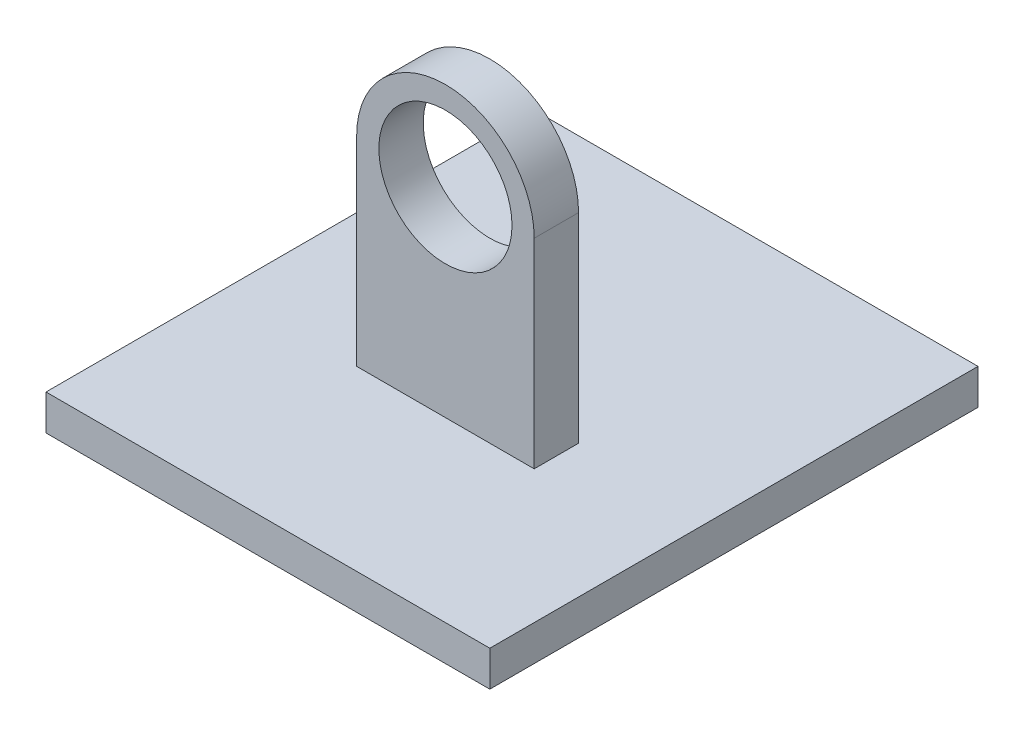
SolidWorks part; units mm, degrees
ref_plane "Front Plane" through (0, 0, 0) normal (0, 0, 1) x (1, 0, 0)
ref_plane "Top Plane" through (0, 0, 0) normal (0, 1, 0) x (1, 0, 0)
ref_plane "Right Plane" through (0, 0, 0) normal (1, 0, 0) x (0, 0, -1)
sketch "Sketch1" plane through (0, 0, 0) normal (0, 0, 1) x (1, 0, 0)
  line L0 (119, -40) -> (119, -108.669) construction
  line L1 (134, -40) -> (134, -80) construction
  line L2 (104, -40) -> (104, -80) construction
  line L3 (134, -80) -> (104, -80) construction
  line L4 (164, -80) -> (74, -80) construction
  line L5 (139, -40) -> (139, -85)
  line L6 (139, -85) -> (99, -85)
  line L7 (99, -40) -> (99, -85)
  arc A0 (134, -40) -> (104, -40) centre (119, -40) ccw construction
  circle A2 centre (119, -40) radius 15 construction
  arc A3 (139, -40) -> (99, -40) centre (119, -40) ccw
  circle A4 centre (119, -40) radius 15
  point P3 (119, -74.3345)
  dimension "D1" = 5
extrude "Boss-Extrude1" add sketch "Sketch1" against normal blind 10
sketch "Sketch2" plane through (0, -85, 0) normal (0, -1, 0) x (1, 0, 0)
  line L1 (169, -70) -> (69, -70)
  line L2 (169, -70) -> (169, 40)
  line L3 (169, 40) -> (69, 40)
  line L4 (69, -70) -> (69, 40)
  line L9 (174, 20) -> (64, 20) construction
  line L10 (174, -330) -> (174, 20) construction
  line L11 (64, 20) -> (64, -330) construction
  dimension "D1" = 20
  dimension "D2" = 110
  dimension "D3" = 5
  dimension "D4" = 5
extrude "Boss-Extrude2" add sketch "Sketch2" along normal blind 10
chamfer "Chamfer1" distance 2 angle 45 4 edges at (119, -95, -70) (69, -95, -15) (119, -95, 40) (169, -95, -15)
